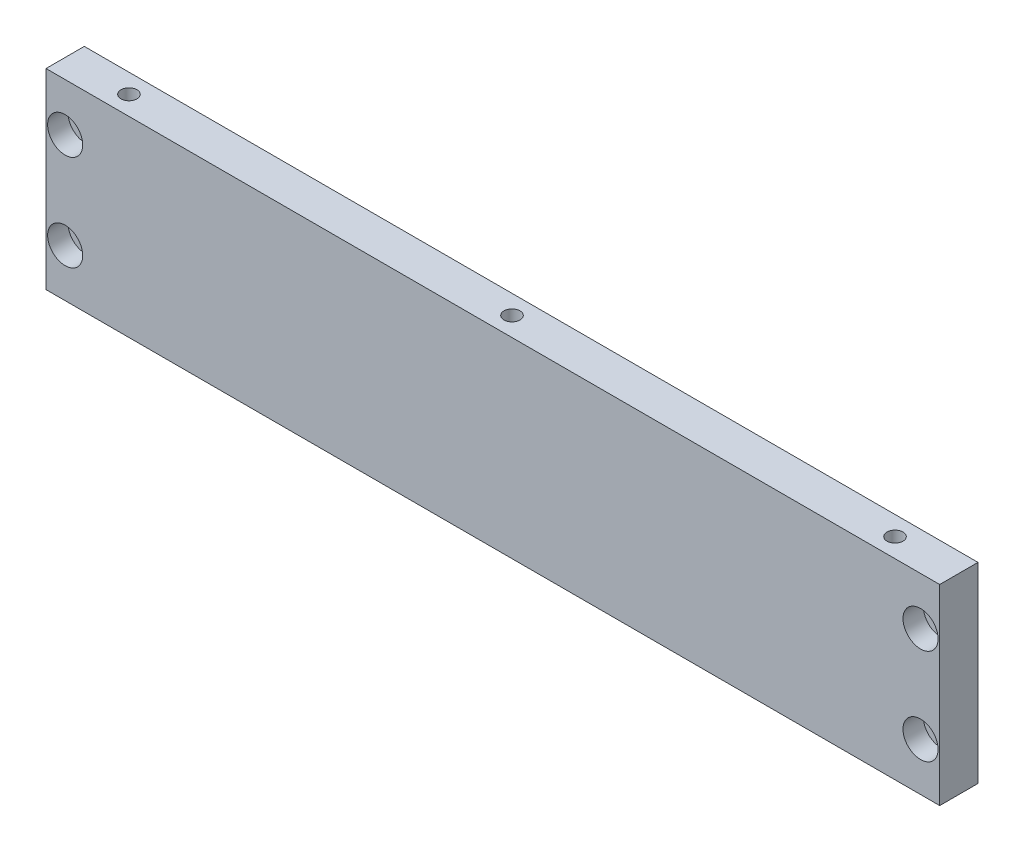
from build123d import *

# Parameters (mm, degrees)
SKETCH_1_W                     = 280
SKETCH_1_H                     = 60
EXTRUDE_1_DEPTH                = 12
HOLE_WIZARD_M6_1_D             = 5
HOLE_WIZARD_M6_1_DEPTH         = 15
HOLE_WIZARD_M6_1_TIP           = 1.502151548
HOLE_WIZARD_M6_2_D             = 5
HOLE_WIZARD_M6_2_DEPTH         = 15
HOLE_WIZARD_M6_2_TIP           = 1.502151548
HOLE_WIZARD_M6_1_2_D           = 6.6
HOLE_WIZARD_M6_1_2_CBORE_D     = 11
HOLE_WIZARD_M6_1_2_CBORE_DEPTH = 6.4


with BuildPart() as part:
    # 草图1 → 凸台-拉伸1 (new body)
    with BuildSketch(Plane.XY):
        with Locations((140, -30)):
            Rectangle(SKETCH_1_W, SKETCH_1_H)
    extrude(amount=EXTRUDE_1_DEPTH)

    # Hole Wizard M6 _1
    with Locations(Plane(origin=(0, 0, 0), x_dir=(1, 0, 0), z_dir=(0, 1, 0))):
        with Locations((260, -6), (140, -6), (20, -6)):
            Hole(HOLE_WIZARD_M6_1_D / 2, depth=HOLE_WIZARD_M6_1_DEPTH)
            with Locations((0, 0, -(HOLE_WIZARD_M6_1_DEPTH + HOLE_WIZARD_M6_1_TIP / 2))):  # 118° drill point
                Cone(0, HOLE_WIZARD_M6_1_D / 2, HOLE_WIZARD_M6_1_TIP, mode=Mode.SUBTRACT)

    # M6 螺纹孔2
    with Locations(Plane(origin=(0, -60, 0), x_dir=(-1, 0, 0), z_dir=(0, -1, 0))):
        with Locations((-260, -6), (-140, -6), (-20, -6)):
            Hole(HOLE_WIZARD_M6_2_D / 2, depth=HOLE_WIZARD_M6_2_DEPTH)
            with Locations((0, 0, -(HOLE_WIZARD_M6_2_DEPTH + HOLE_WIZARD_M6_2_TIP / 2))):  # 118° drill point
                Cone(0, HOLE_WIZARD_M6_2_D / 2, HOLE_WIZARD_M6_2_TIP, mode=Mode.SUBTRACT)

    # Hole Wizard M6 _1 2 (through all)
    with Locations(Plane.XY.offset(12)):
        with Locations((274, -45), (274, -15), (6, -45), (6, -15)):
            CounterBoreHole(HOLE_WIZARD_M6_1_2_D / 2, HOLE_WIZARD_M6_1_2_CBORE_D / 2, HOLE_WIZARD_M6_1_2_CBORE_DEPTH)


solid = part.part
